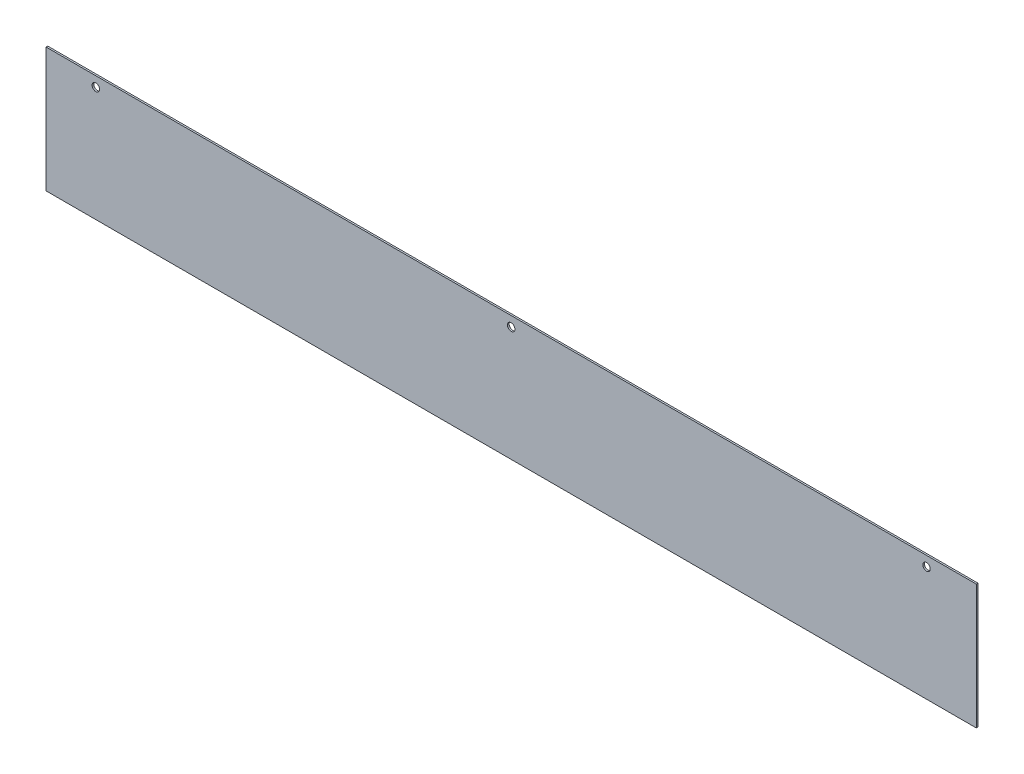
SolidWorks part; units mm, degrees
material "45#"
ref_plane "Front Plane" through (0, 0, 0) normal (0, 0, 1) x (1, 0, 0)
ref_plane "Top Plane" through (0, 0, 0) normal (0, 1, 0) x (1, 0, 0)
ref_plane "Right Plane" through (0, 0, 0) normal (1, 0, 0) x (0, 0, -1)
sketch "Sketch1" plane through (0, 0, 0) normal (0, 1, 0) x (1, 0, 0)
  line L0 (280, 0.5) -> (-280, -0.5) construction
  line L1 (-280, 0.5) -> (280, 0.5)
  line L2 (-280, 0.5) -> (-280, -0.5)
  line L3 (-280, -0.5) -> (280, -0.5)
  line L4 (280, 0.5) -> (280, -0.5)
  dimension "D1" = 560
  dimension "D2" = 1
extrude "Extrude1" add sketch "Sketch1" along normal mid plane 75
sketch "Sketch3" plane through (0, 0, 0.5) normal (0, 0, 1) x (1, 0, 0)
  line L0 (0, 37.5) -> (0, -37.5) construction
  line L1 (-280, 37.5) -> (280, 37.5) construction
  line L2 (-280, -37.5) -> (280, -37.5) construction
  line L3 (-250, 31.5) -> (0, 31.5) construction
  circle A1 centre (-250, 31.5) radius 2.25
  circle A2 centre (250, 31.5) radius 2.25
  circle A4 centre (0, 31.5) radius 2.25
  dimension "D1" = 4.5
  dimension "D2" = 6
  dimension "D3" = 500
extrude "Cut-Extrude1" cut sketch "Sketch3" against normal through all
